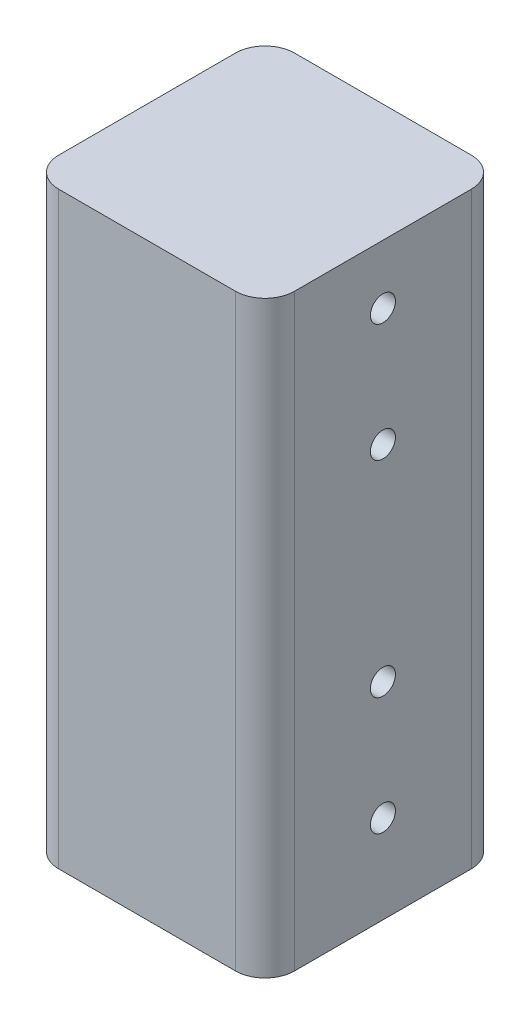
from build123d import *

# Parameters (mm, degrees)
SKETCH1_W                      = 80
SKETCH1_H                      = 199.7
BOSS_EXTRUDE1_DEPTH            = 80
F_8_5_8_5_DIAMETER_HOLE1_D     = 8.5
F_8_5_8_5_DIAMETER_HOLE1_DEPTH = 20
F_8_5_8_5_DIAMETER_HOLE1_TIP   = 2.553657631
FILLET2_R                      = 10
SKETCH5_R                      = 13
CUT_EXTRUDE1_DEPTH             = 100
F_8_5_8_5_DIAMETER_HOLE2_D     = 8.5
F_8_5_8_5_DIAMETER_HOLE2_DEPTH = 20
F_8_5_8_5_DIAMETER_HOLE2_TIP   = 2.553657631


with BuildPart() as part:
    # Sketch1 → Boss-Extrude1 (new body)
    with BuildSketch(Plane(origin=(0, 0, -30), x_dir=(-1, 0, 0), z_dir=(0, 0, -1))):
        with Locations((0, 99.85)):
            Rectangle(SKETCH1_W, SKETCH1_H)
    extrude(amount=-BOSS_EXTRUDE1_DEPTH)

    # Ø8.5 (8.5) Diameter Hole1
    with Locations(Plane(origin=(40, 0, 0), x_dir=(0, 0, -1), z_dir=(1, 0, 0))):
        with Locations((-10, 30), (-10, 179.7), (-10, 70)):
            Hole(F_8_5_8_5_DIAMETER_HOLE1_D / 2, depth=F_8_5_8_5_DIAMETER_HOLE1_DEPTH)
            with Locations((0, 0, -(F_8_5_8_5_DIAMETER_HOLE1_DEPTH + F_8_5_8_5_DIAMETER_HOLE1_TIP / 2))):  # 118° drill point
                Cone(0, F_8_5_8_5_DIAMETER_HOLE1_D / 2, F_8_5_8_5_DIAMETER_HOLE1_TIP, mode=Mode.SUBTRACT)

    # Fillet2
    fillet2_edges = [part.edges().sort_by_distance(p)[0] for p in [
        (-40, 99.85, 50),
        (40, 99.85, 50),
        (-40, 99.85, -30),
        (40, 99.85, -30),
    ]]
    fillet(fillet2_edges, radius=FILLET2_R)

    # Sketch5 → Cut-Extrude1 (cut)
    with BuildSketch(Plane.XZ):
        with Locations((0, 10)):
            Circle(SKETCH5_R)
    extrude(amount=-CUT_EXTRUDE1_DEPTH, mode=Mode.SUBTRACT)

    # Ø8.5 (8.5) Diameter Hole2
    with Locations(Plane(origin=(40, 0, 0), x_dir=(0, 0, -1), z_dir=(1, 0, 0))):
        with Locations((-10, 139.7)):
            Hole(F_8_5_8_5_DIAMETER_HOLE2_D / 2, depth=F_8_5_8_5_DIAMETER_HOLE2_DEPTH)
            with Locations((0, 0, -(F_8_5_8_5_DIAMETER_HOLE2_DEPTH + F_8_5_8_5_DIAMETER_HOLE2_TIP / 2))):  # 118° drill point
                Cone(0, F_8_5_8_5_DIAMETER_HOLE2_D / 2, F_8_5_8_5_DIAMETER_HOLE2_TIP, mode=Mode.SUBTRACT)


solid = part.part
